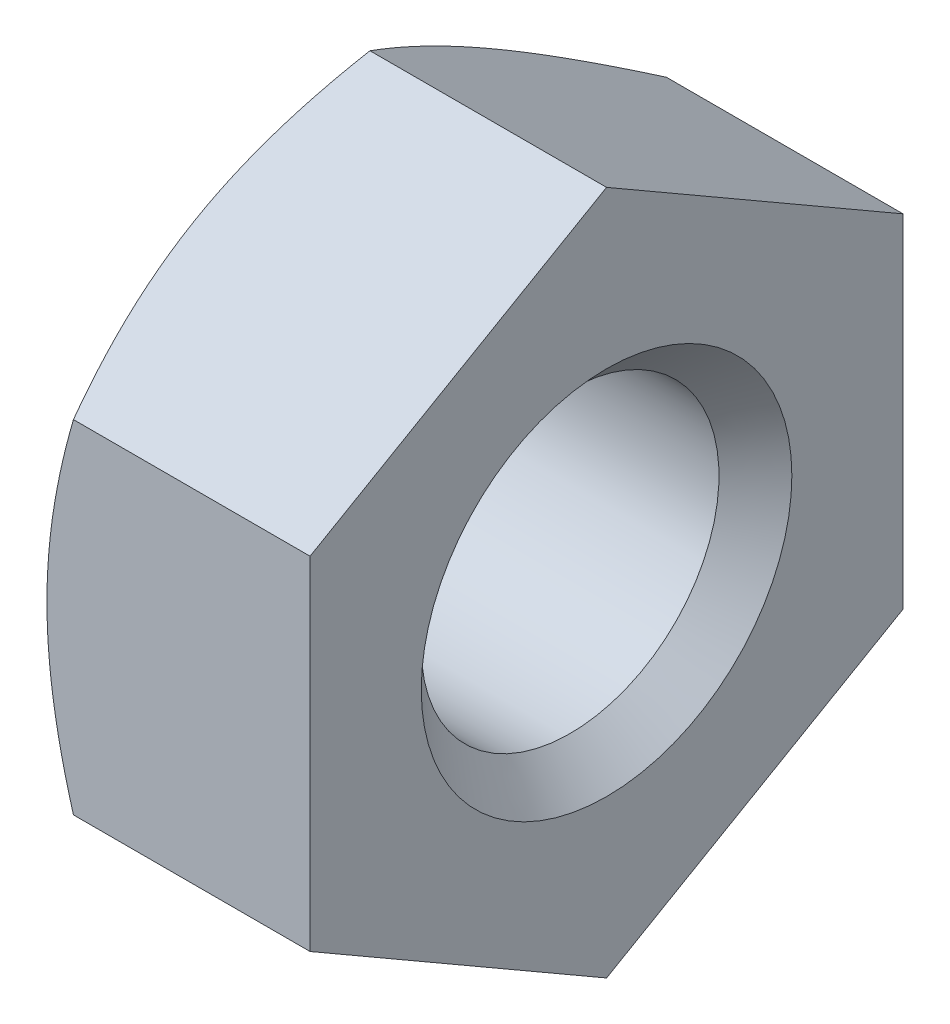
SolidWorks part; units mm, degrees
ref_plane "Front Plane" through (0, 0, 0) normal (0, 0, 1) x (1, 0, 0)
ref_plane "Top Plane" through (0, 0, 0) normal (0, 1, 0) x (1, 0, 0)
ref_plane "Right Plane" through (0, 0, 0) normal (1, 0, 0) x (0, 0, -1)
sketch "Sketch1" plane through (0, 0, 0) normal (0, 0, 1) x (1, 0, 0)
  line L0 (-4, 0) -> (-4, 3.22)
  line L1 (-4, 3.22) -> (-2.9377, 5.06)
  line L2 (-2.9377, 5.06) -> (0, 5.06)
  line L3 (0, 5.06) -> (0, 0)
  line L4 (0, 0) -> (-4, 0)
  line L5 (0, 0) -> (-4, 0) construction
revolve "Revolve1" add sketch "Sketch1" angle 360 about L5
sketch "Sketch2" plane through (0, 0, 0) normal (0, 0, 1) x (1, 0, 0)
  line L0 (-4, 0) -> (-4, 2.5)
  line L1 (-4, 2.5) -> (-3.5085, 2.0085)
  line L2 (-3.5085, 2.0085) -> (-0.4915, 2.0085)
  line L3 (-0.4915, 2.0085) -> (0, 2.5)
  line L4 (0, 2.5) -> (0, 0)
  line L5 (0, 0) -> (-4, 0)
  line L6 (0, 0) -> (-4, 0) construction
revolve "Cut-Revolve1" cut sketch "Sketch2" angle 360 about L6
cosmetic thread "Cosmetic Thread1" parameters "D1"=4, "D2"=5
sketch "Sketch3" plane through (0, 0, 0) normal (1, 0, 0) x (0, 0, -1)
  line L0 (-8, -8) -> (8, -8)
  line L1 (8, -8) -> (8, 8)
  line L2 (8, 8) -> (-8, 8)
  line L3 (-8, 8) -> (-8, -8)
  line L4 (-4, 2.3094) -> (-4, -2.3094)
  line L5 (-4, -2.3094) -> (0, -4.6188)
  line L6 (0, -4.6188) -> (4, -2.3094)
  line L7 (4, -2.3094) -> (4, 2.3094)
  line L8 (4, 2.3094) -> (0, 4.6188)
  line L9 (0, 4.6188) -> (-4, 2.3094)
extrude "Cut-Extrude1" cut sketch "Sketch3" against normal blind 4
